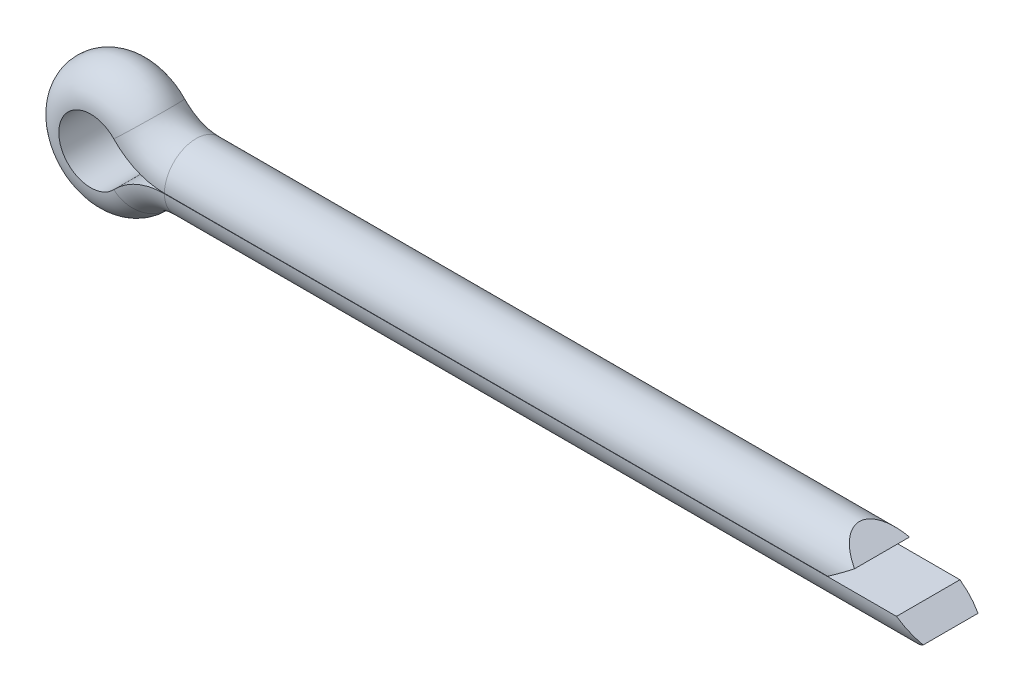
SolidWorks part; units mm, degrees
ref_plane "前视基准面" through (0, 0, 0) normal (0, 0, 1) x (1, 0, 0)
ref_plane "上视基准面" through (0, 0, 0) normal (0, 1, 0) x (1, 0, 0)
ref_plane "右视基准面" through (0, 0, 0) normal (1, 0, 0) x (0, 0, -1)
sketch "尺寸草图" plane through (0, 0, 0) normal (0, 0, 1) x (1, 0, 0)
  line L0 (44.3, 1.85) -> (4.3, 1.85)
  line L1 (4.3, -1.85) -> (48.3, -1.85)
  line L2 (4.3, 0) -> (27.3859, 0) construction
  line L3 (4.3, 0) -> (4.3, -0.0723) construction
  line L4 (-3.7, 0) -> (-3.7, 18.8979) construction
  arc A0 (4.3, 1.85) -> (2.6865, 2.5442) centre (4.3, 4.0723) cw
  arc A1 (2.6865, 2.5442) -> (2.6865, -2.5442) centre (0, 0) ccw
  arc A2 (2.6865, -2.5442) -> (4.3, -1.85) centre (4.3, -4.0723) cw
  dimension "c" = 7.4
  dimension "d1" = 3.7
  dimension "b" = 8
  dimension "l" = 40
  dimension "a" = 4
ref_plane "基准面1" through (44.3, 1.85, 0) normal (-1, 0, 0) x (0, 0, 1)
sketch "草图2" plane through (44.3, 1.85, 0) normal (-1, 0, 0) x (0, 0, 1)
  line L0 (0, -5.55) -> (0, 1.85) construction
  line L1 (-1.85, -1.84) -> (1.85, -1.84)
  arc A0 (1.85, -1.84) -> (-1.85, -1.84) centre (0, -1.85) ccw
  dimension "d" = 3.7
  dimension "D1" = 0.01
sweep "扫描2" add profiles "草图2" path "尺寸草图"
sketch "草图3" plane through (0, 0, 0) normal (0, 0, 1) x (1, 0, 0)
  line L0 (4.3, 0) -> (4.3, 16.2682) construction
  line L1 (4.3, 0) -> (37.4999, 0) construction
  line L2 (48.3, -1.85) -> (48.3, -0.01) construction
  line L3 (44.3, 0.92) -> (42.9825, 1.85)
  line L4 (44.3, 1.85) -> (4.3, 1.85) construction
  line L5 (4.3, -1.85) -> (48.3, -1.85) construction
  line L6 (44.3, 0.92) -> (42.9755, 0)
  line L7 (48.3, -0.93) -> (46.9825, 0)
  line L9 (48.3, -0.93) -> (46.9755, -1.85)
  line L10 (46.9825, 0) -> (42.9755, 0)
  line L11 (42.9825, 1.85) -> (48.31, 1.85)
  line L12 (48.31, 1.85) -> (48.31, -1.85)
  line L13 (48.31, -1.85) -> (46.9755, -1.85)
  line L14 (44.3, 1.85) -> (44.3, 0.01) construction
  dimension "D1" = 0.01
  dimension "D3" = 70
  dimension "D4" = 70
extrude "切除-拉伸1" cut sketch "草图3" against normal through all and the other way through all
